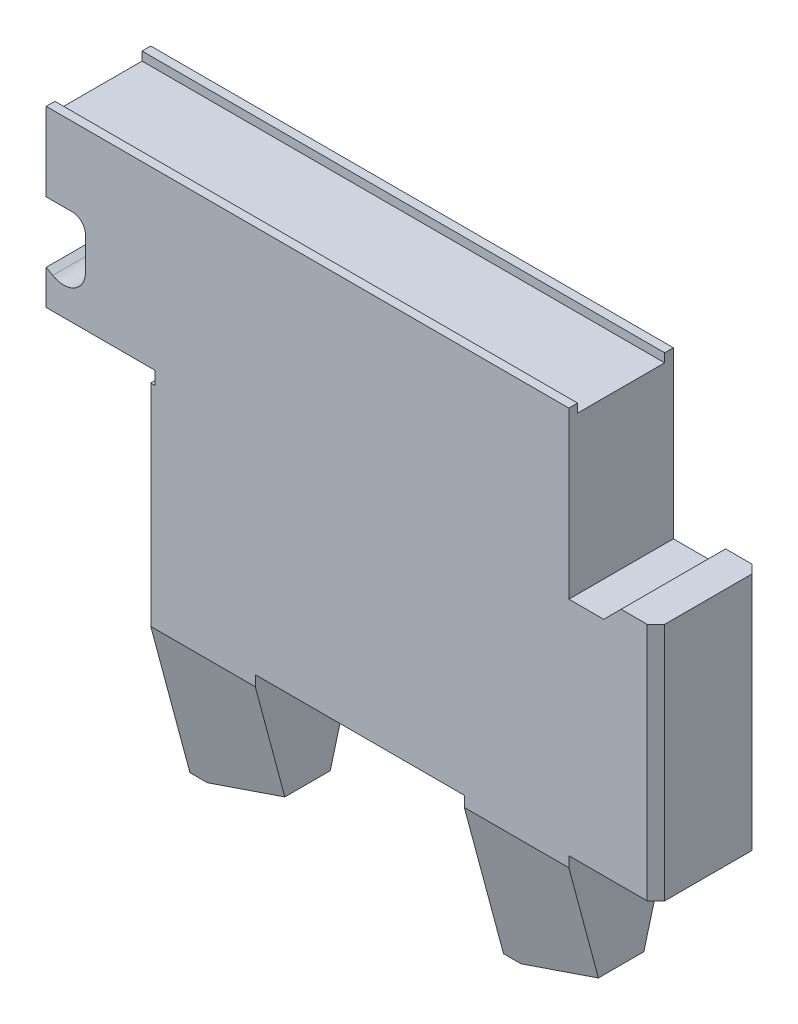
from build123d import *

# Parameters (mm, degrees)
EXTRUDE_1_DEPTH     = 6
CUT_EXTRUDE_1_DEPTH = 73.154348448
SKETCH_5_W          = 60
SKETCH_5_H          = 10
CUT_EXTRUDE_2_DEPTH = 1
CHAMFER_1_SIZE      = 1


with BuildPart() as part:
    # 草图1 → 凸台-拉伸1 (new, symmetric)
    with BuildSketch(Plane.XY):
        with BuildLine():
            Line((0, 0), (0, 4))
            Line((0, 4), (0.75, 3.566987298))
            ThreePointArc((0.75, 3.566987298), (3.25, 3.566987298), (4.5, 5.732050808))
            Line((4.5, 5.732050808), (4.5, 9.5))
            ThreePointArc((4.5, 9.5), (4.060660172, 10.560660172), (3, 11))
            Line((3, 11), (0, 11))
            Line((0, 11), (0, 20))
            Line((0, 20), (60, 20))
            Line((60, 20), (60, 1))
            Line((60, 1), (64, 1))
            Line((64, 1), (66, 3))
            Line((66, 3), (70, 3))
            Line((70, 3), (70, -24.5))
            Line((70, -24.5), (60, -24.5))
            Line((60, -24.5), (60, -38.357864376))
            Line((60, -38.357864376), (50, -42.5))
            Line((50, -42.5), (48, -42.5))
            Line((48, -42.5), (48, -24.5))
            Line((48, -24.5), (24, -24.5))
            Line((24, -24.5), (24, -38.357864376))
            Line((24, -38.357864376), (14, -42.5))
            Line((14, -42.5), (12, -42.5))
            Line((12, -42.5), (12, -1.5))
            Line((12, -1.5), (12.5, -1.5))
            Line((12.5, -1.5), (12.5, 0))
            Line((12.5, 0), (0, 0))
        make_face()
    extrude(amount=EXTRUDE_1_DEPTH, both=True)

    # 草图2 → 切除-拉伸1 (cut, through all)
    with BuildSketch(Plane.ZY.offset(-12)):
        Polygon((6, -25.705771366), (6, -47.5), (-6, -47.5), (-6, -25.705771366), (-1.5, -42.5), (1.5, -42.5), align=None)
    extrude(amount=-CUT_EXTRUDE_1_DEPTH, mode=Mode.SUBTRACT)

    # 草图5 → 切除-拉伸2 (cut)
    with BuildSketch(Plane(origin=(0, 20, 0), x_dir=(1, 0, 0), z_dir=(0, 1, 0))):
        with Locations((30, 0)):
            Rectangle(SKETCH_5_W, SKETCH_5_H)
    extrude(amount=-CUT_EXTRUDE_2_DEPTH, mode=Mode.SUBTRACT)

    # 倒角1
    chamfer_1_edges = [part.edges().sort_by_distance(p)[0] for p in [
        (70, -10.75, -6),
        (70, -10.75, 6),
    ]]
    chamfer(chamfer_1_edges, length=CHAMFER_1_SIZE)


solid = part.part
